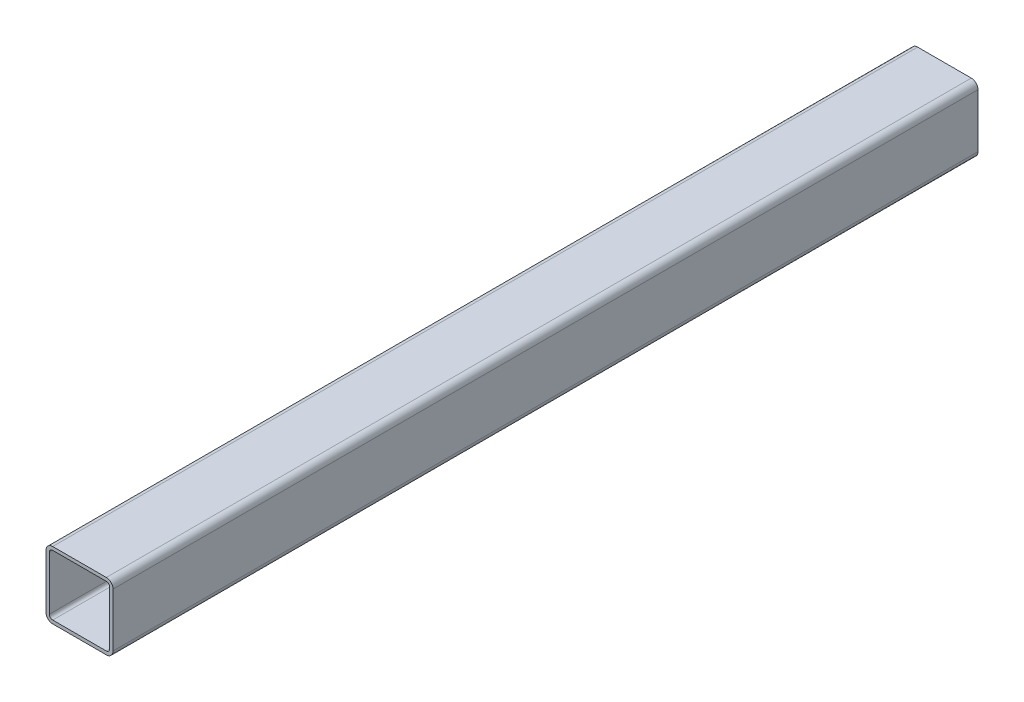
from build123d import *

# Parameters (mm, degrees)
BOSS_EXTRUDE_1_DEPTH = 645


with BuildPart() as part:
    # Sketch 1 → Boss-Extrude 1 (new, symmetric)
    with BuildSketch(Plane.XY):
        with BuildLine():
            Line((0, 50), (-40, 50))
            ThreePointArc((-40, 50), (-47.071067812, 47.071067812), (-50, 40))
            Line((-50, 40), (-50, 0))
            Line((-50, 0), (-50, -40))
            ThreePointArc((-50, -40), (-47.071067812, -47.071067812), (-40, -50))
            Line((-40, -50), (40, -50))
            ThreePointArc((40, -50), (47.071067812, -47.071067812), (50, -40))
            Line((50, -40), (50, 0))
            Line((50, 0), (50, 40))
            ThreePointArc((50, 40), (47.071067812, 47.071067812), (40, 50))
            Line((40, 50), (0, 50))
        make_face()
        with BuildLine():
            Line((0, 45), (-40, 45))
            ThreePointArc((-40, 45), (-43.535533906, 43.535533906), (-45, 40))
            Line((-45, 40), (-45, 0))
            Line((-45, 0), (-45, -40))
            ThreePointArc((-45, -40), (-43.535533906, -43.535533906), (-40, -45))
            Line((-40, -45), (40, -45))
            ThreePointArc((40, -45), (43.535533906, -43.535533906), (45, -40))
            Line((45, -40), (45, 0))
            Line((45, 0), (45, 40))
            ThreePointArc((45, 40), (43.535533906, 43.535533906), (40, 45))
            Line((40, 45), (0, 45))
        make_face(mode=Mode.SUBTRACT)
    extrude(amount=BOSS_EXTRUDE_1_DEPTH, both=True)


solid = part.part
